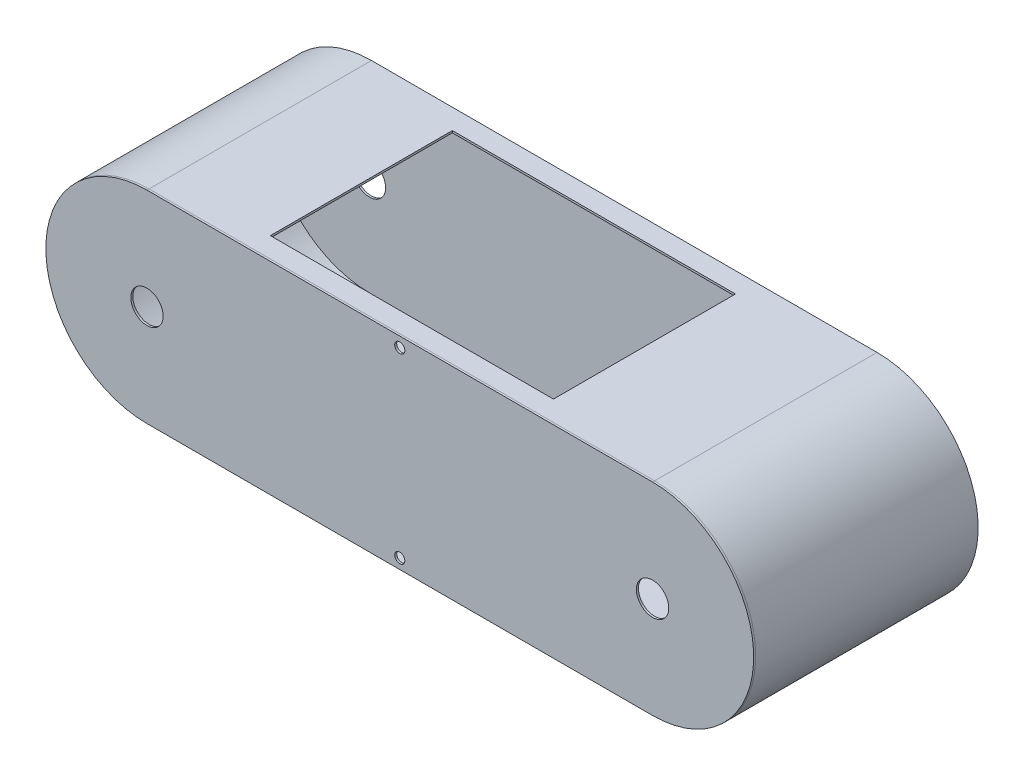
from build123d import *

# Parameters (mm, degrees)
EXTRUDE_1_DEPTH     = 110
SHELL_1_T           = -1
EXTRUDE_2_DEPTH     = 1
SKETCH_3_R          = 8
CUT_EXTRUDE_1_DEPTH = 324.760714108
SKETCH_5_R          = 2.5
CUT_EXTRUDE_2_DEPTH = 3
SKETCH_6_W          = 80
SKETCH_6_H          = 90
CUT_EXTRUDE_3_DEPTH = 3
SKETCH_7_W          = 140
SKETCH_7_H          = 90
CUT_EXTRUDE_4_DEPTH = 3


with BuildPart() as part:
    # 草图1 → 凸台-拉伸1 (new body)
    with BuildSketch(Plane.XY):
        with BuildLine():
            Line((0, 50), (250, 50))
            ThreePointArc((250, 50), (300, 0), (250, -50))
            Line((250, -50), (0, -50))
            ThreePointArc((0, -50), (-50, 0), (0, 50))
        make_face()
    extrude(amount=EXTRUDE_1_DEPTH)

    # 抽壳1
    shell_1_openings = [part.faces().sort_by_distance(p)[0] for p in [
        (125, 0, 110),
    ]]
    offset(amount=SHELL_1_T, openings=shell_1_openings, kind=Kind.INTERSECTION)


with BuildPart() as body_2:
    # 草图2 → 凸台-拉伸2 (new body)
    with BuildSketch(Plane.XY.offset(110)):
        with BuildLine():
            Line((0, -50), (250, -50))
            ThreePointArc((250, -50), (300, 0), (250, 50))
            Line((250, 50), (0, 50))
            ThreePointArc((0, 50), (-50, 0), (0, -50))
        make_face()
    extrude(amount=EXTRUDE_2_DEPTH)


with BuildPart() as cut_extrude_1_tool:
    # 草图3 → 切除-拉伸1 (new, through all)
    with BuildSketch(Plane.XY.offset(111)):
        Circle(SKETCH_3_R)
        with Locations((250, 0)):
            Circle(SKETCH_3_R)
    extrude(amount=-CUT_EXTRUDE_1_DEPTH)


with BuildPart() as part_1:
    add(part.part)

    # 切除-拉伸1: cut by cut_extrude_1_tool
    add(cut_extrude_1_tool.part, mode=Mode.SUBTRACT)

    # 草图6 → 切除-拉伸3 (cut)
    with BuildSketch(Plane.XZ.offset(50)):
        with Locations((95, 55)):
            Rectangle(SKETCH_6_W, SKETCH_6_H)
    extrude(amount=-CUT_EXTRUDE_3_DEPTH, mode=Mode.SUBTRACT)

    # 草图7 → 切除-拉伸4 (cut)
    with BuildSketch(Plane(origin=(0, 50, 0), x_dir=(1, 0, 0), z_dir=(0, 1, 0))):
        with Locations((120, -55)):
            Rectangle(SKETCH_7_W, SKETCH_7_H)
    extrude(amount=-CUT_EXTRUDE_4_DEPTH, mode=Mode.SUBTRACT)


with BuildPart() as body_2_1:
    add(body_2.part)

    # 切除-拉伸1: cut by cut_extrude_1_tool
    add(cut_extrude_1_tool.part, mode=Mode.SUBTRACT)

    # 草图5 → 切除-拉伸2 (cut)
    with BuildSketch(Plane.XY.offset(111)):
        with Locations((-100, 45)):
            Circle(SKETCH_5_R)
        with Locations((350, 45)):
            Circle(SKETCH_5_R)
        with Locations((-100, -45)):
            Circle(SKETCH_5_R)
        with Locations((350, -45)):
            Circle(SKETCH_5_R)
        with Locations((420, 0)):
            Circle(SKETCH_5_R)
        with Locations((-170, 0)):
            Circle(SKETCH_5_R)
        with Locations((125, 45)):
            Circle(SKETCH_5_R)
        with Locations((125, -45)):
            Circle(SKETCH_5_R)
    extrude(amount=-CUT_EXTRUDE_2_DEPTH, mode=Mode.SUBTRACT)


solid = Compound([part_1.part, body_2_1.part])
